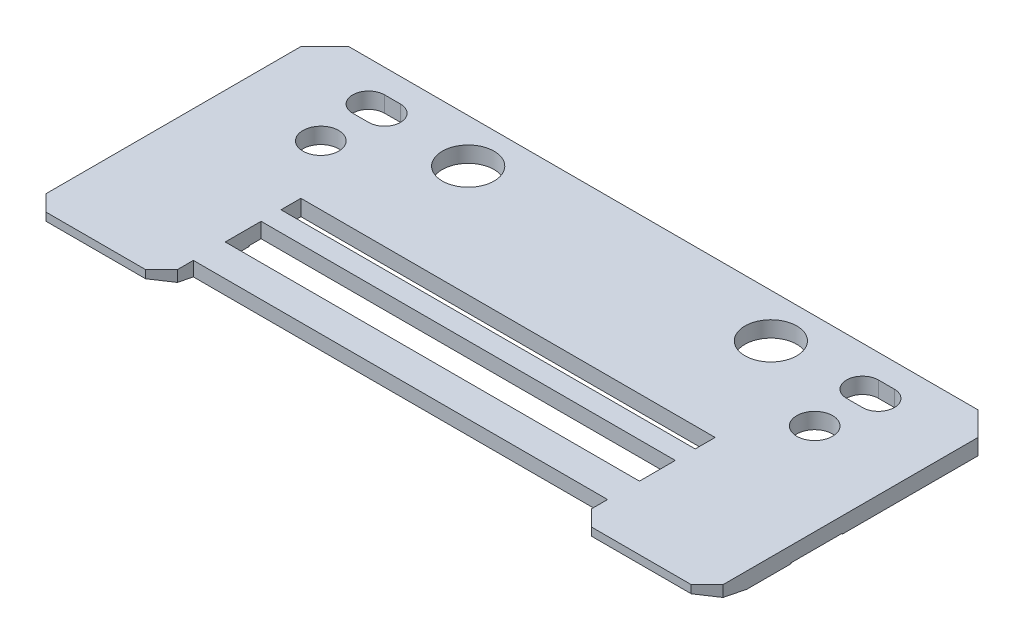
SolidWorks part; units mm, degrees
ref_plane "Front Plane" through (0, 0, 0) normal (0, 0, 1) x (1, 0, 0)
ref_plane "Top Plane" through (0, 0, 0) normal (0, 1, 0) x (1, 0, 0)
ref_plane "Right Plane" through (0, 0, 0) normal (1, 0, 0) x (0, 0, -1)
sketch "Sketch1" plane through (0, 0, 0) normal (0, 1, 0) x (1, 0, 0)
  line L1 (-42.5, 22.5) -> (42.5, 22.5)
  line L2 (-42.5, 22.5) -> (-42.5, -22.5)
  line L3 (-42.5, -22.5) -> (42.5, -22.5)
  line L4 (42.5, 22.5) -> (42.5, -22.5)
  line L5 (-42.5, 22.5) -> (42.5, -22.5) construction
  line L6 (-42.5, -22.5) -> (42.5, 22.5) construction
  point P0 (0, 0)
  dimension "D1" = 85
  dimension "D2" = 45
extrude "Boss-Extrude1" add sketch "Sketch1" along normal blind 2
sketch "Sketch2" plane through (0, 2, 0) normal (0, 1, 0) x (1, 0, 0)
  line L0 (0, 0) -> (0, -50000) construction
  line L1 (-42.5, -22.5) -> (42.5, -22.5) construction
  line L2 (-26, -10.5) -> (26, -10.5)
  line L3 (-26, -10.5) -> (-26, -22.5)
  line L4 (-26, -22.5) -> (26, -22.5)
  line L5 (26, -10.5) -> (26, -22.5)
  line L6 (-26, -10.5) -> (26, -22.5) construction
  line L7 (-26, -22.5) -> (26, -10.5) construction
  line L8 (-26, -7.5) -> (-26, 49992.5) construction
  line L9 (26, -7.5) -> (26, 49992.5) construction
  line L10 (42.5, 22.5) -> (-42.5, 22.5) construction
  line L11 (-26, -6.5) -> (26, -6.5)
  line L12 (-26, -6.5) -> (-26, -2)
  line L13 (-26, -2) -> (26, -2)
  line L14 (26, -6.5) -> (26, -2)
  line L15 (-26, 0.5) -> (26, 0.5)
  line L16 (-26, 0.5) -> (-26, 3)
  line L17 (-26, 3) -> (26, 3)
  line L18 (26, 0.5) -> (26, 3)
  line L19 (-26, 22.5) -> (26, 22.5)
  line L20 (-26, 22.5) -> (-26, 8.7)
  line L21 (-26, 8.7) -> (26, 8.7)
  line L22 (26, 22.5) -> (26, 8.7)
  point P3 (0, -16.5)
  dimension "D1" = 52
  dimension "D2" = 12
  dimension "D3" = 4.5
  dimension "D4" = 2.5
  dimension "D5" = 16
  dimension "D6" = 23
  dimension "D7" = 13.8
extrude "Cut-Extrude1" cut sketch "Sketch2" against normal blind 10
sketch "Sketch3" plane through (0, 2, 0) normal (0, 1, 0) x (1, 0, 0)
  line L0 (-42.5, 22.5) -> (-42.5, -22.5) construction
  line L1 (42.5, 22.5) -> (-42.5, 22.5)
  line L2 (42.5, 22.5) -> (42.5, 8.7)
  line L3 (42.5, 8.7) -> (-42.5, 8.7)
  line L4 (-42.5, 22.5) -> (-42.5, 8.7)
  line L5 (-26, 8.7) -> (26, 8.7) construction
extrude "Cut-Extrude2" cut sketch "Sketch3" against normal blind 10
sketch "Sketch5" plane through (0, 0, 0) normal (0, -1, 0) x (1, 0, 0)
  line L0 (42.5, 22.5) -> (42.5, -8.7) construction
  line L1 (42.5, -2) -> (-42.5, -2)
  line L2 (42.5, -2) -> (42.5, 3.5)
  line L3 (42.5, 3.5) -> (-42.5, 3.5)
  line L4 (-42.5, -2) -> (-42.5, 3.5)
  line L5 (-42.5, -8.7) -> (-42.5, 22.5) construction
  dimension "D2" = 5.5
extrude "Cut-Extrude4" cut sketch "Sketch5" against normal blind 0.1
chamfer "Chamfer2" distance 0.5 distance2 2 1 edges at (42.5, 0.05, 3.5)
chamfer "Chamfer3" distance 2 distance2 0.5 1 edges at (42.5, 0.05, -2)
sketch "Sketch8" plane through (0, 2, 0) normal (0, 1, 0) x (1, 0, 0)
  line L0 (42.5, -22.5) -> (42.5, 8.7) construction
  line L1 (-42.5, 8.7) -> (42.5, 8.7)
  line L2 (-42.5, 8.7) -> (-42.5, 22.5)
  line L3 (-42.5, 22.5) -> (42.5, 22.5)
  line L4 (42.5, 8.7) -> (42.5, 22.5)
  dimension "D1" = 13.8
extrude "Boss-Extrude2" add sketch "Sketch8" against normal up to surface (2 mm away) up to face at (4.5, 0, -3.7667)
chamfer "Chamfer4" distance 3 angle 45 2 edges at (42.5, 1, -22.5) (-42.5, 1, -22.5)
sketch "Sketch6" plane through (0, 2, 0) normal (0, 1, 0) x (1, 0, 0)
  line L2 (39.5, 22.5) -> (-39.5, 22.5) construction
  line L3 (0, 22.5) -> (0, -49977.5) construction
  circle A0 centre (-31, 17.5) radius 2
  circle A1 centre (31, 17.5) radius 2
  point P4 (0, 22.5)
  dimension "D1" = 4
  dimension "D2" = 62
  dimension "D3" = 5
extrude "Cut-Extrude5" cut sketch "Sketch6" against normal blind 10
sketch "Sketch7" plane through (0, 2, 0) normal (0, 1, 0) x (1, 0, 0)
  line L0 (31, -8.5) -> (31, 49991.5) construction
  line L1 (38.062, 17.5) -> (50038.062, 17.5) construction
  line L2 (32, 17.5) -> (30, 17.5) construction
  line L3 (32, 15.5) -> (30, 15.5)
  line L4 (32, 19.5) -> (30, 19.5)
  line L5 (0, 22.5) -> (0, -49977.5) construction
  line L6 (39.5, 22.5) -> (-39.5, 22.5) construction
  line L7 (-32, 17.5) -> (-30, 17.5) construction
  line L8 (-32, 15.5) -> (-30, 15.5)
  line L9 (-32, 19.5) -> (-30, 19.5)
  arc A0 (-32, 15.5) -> (-32, 19.5) centre (-32, 17.5) cw
  arc A1 (32, 15.5) -> (32, 19.5) centre (32, 17.5) ccw
  arc A2 (30, 19.5) -> (30, 15.5) centre (30, 17.5) ccw
  arc A3 (-30, 19.5) -> (-30, 15.5) centre (-30, 17.5) cw
  point P7 (31, 17.5)
  point P16 (0, 22.5)
  point P19 (-31, 17.5)
  dimension "D1" = 4
  dimension "D2" = 2
extrude "Cut-Extrude6" cut sketch "Sketch7" against normal blind 6
sketch "Sketch9" plane through (0, 2, 0) normal (0, 1, 0) x (1, 0, 0)
  circle A0 centre (-19, 17) radius 3.25
  circle A1 centre (19, 17) radius 3.25
  dimension "D1" = 6.5
extrude "Cut-Extrude8" cut sketch "Sketch9" against normal blind 10
sketch "Sketch4" plane through (0, 2, 0) normal (0, 1, 0) x (1, 0, 0)
  line L0 (0, 0) -> (0, -50000) construction
  line L2 (39.5, 22.5) -> (-39.5, 22.5) construction
  circle A0 centre (-31, 10.5) radius 2.25
  circle A1 centre (31, 10.5) radius 2.25
  dimension "D1" = 62
  dimension "D2" = 12
  dimension "D3" = 4.5
extrude "Cut-Extrude3" cut sketch "Sketch4" against normal blind 10
sketch "Sketch10" plane through (0, 2, 0) normal (0, 1, 0) x (1, 0, 0)
  line L0 (42.5, -22.5) -> (42.5, 19.5) construction
  line L1 (-42.5, -22.5) -> (42.5, -22.5)
  line L2 (-42.5, -22.5) -> (-42.5, -14.5)
  line L3 (-42.5, -14.5) -> (42.5, -14.5)
  line L4 (42.5, -22.5) -> (42.5, -14.5)
  dimension "D1" = 8
extrude "Cut-Extrude9" cut sketch "Sketch10" against normal blind 10
chamfer "Chamfer5" distance 1 distance2 5 1 edges at (-34.25, 0, 14.5)
chamfer "Chamfer6" distance 2 angle 45 4 edges at (42.5, 1.5, 14.5) (26, 1.5, 14.5) (-26, 1.5, 14.5) (-42.5, 1.5, 14.5)
